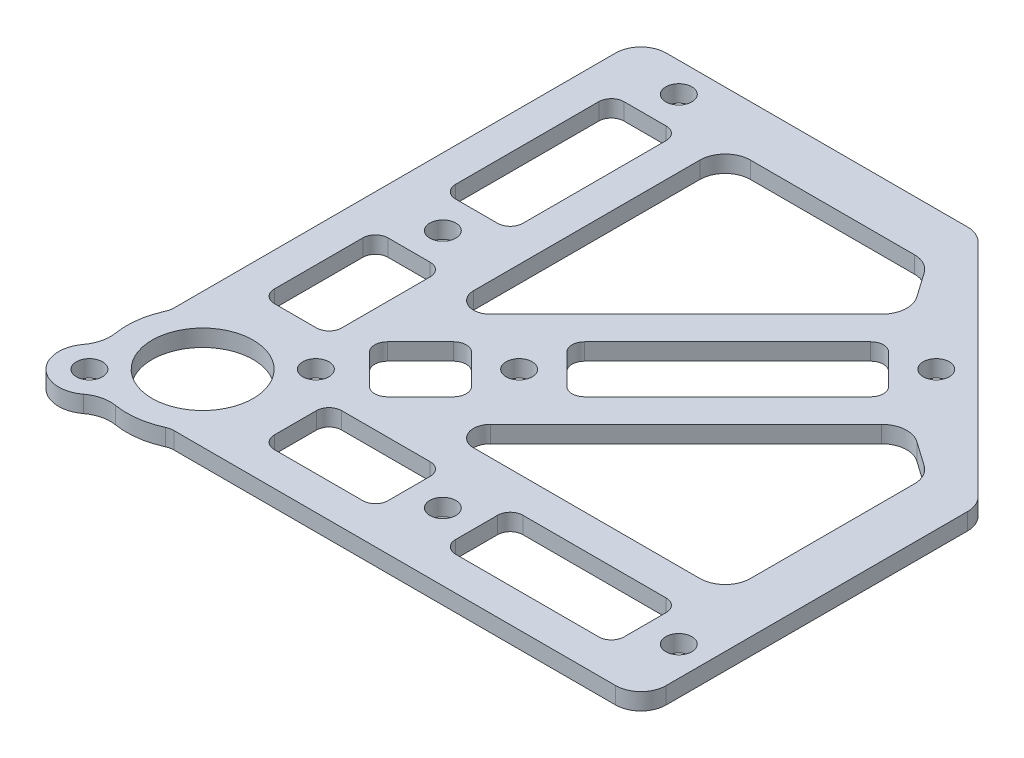
SolidWorks part; units mm, degrees
material "Thornel Mat VMA"
ref_plane "前视基准面" through (0, 0, 0) normal (0, 0, 1) x (1, 0, 0)
ref_plane "上视基准面" through (0, 0, 0) normal (0, 1, 0) x (1, 0, 0)
ref_plane "右视基准面" through (0, 0, 0) normal (1, 0, 0) x (0, 0, -1)
other "Configuration Table"
sketch "草图1" plane through (0, 0, 0) normal (0, 1, 0) x (1, 0, 0)
  line L0 (0, 0) -> (79.3925, 0) construction
  line L1 (0, 0) -> (0, 72.0385) construction
  line L2 (0, 0) -> (60.9542, 60.9542) construction
  line L3 (10.1348, -8) -> (60, -8)
  line L4 (0, 0) -> (-6.7175, 6.7175) construction
  line L5 (60, 32) -> (60, -8)
  line L6 (60, 32) -> (32, 60)
  line L7 (19.3137, 8) -> (54, 8)
  line L8 (54, 8) -> (54, 32)
  line L9 (54, 32) -> (47.7147, 36.401)
  line L10 (47.7147, 36.401) -> (19.3137, 8)
  line L11 (8, 19.3137) -> (8, 54)
  line L12 (32.5, 4) -> (52.5, 4)
  line L13 (32.5, 4) -> (32.5, -4)
  line L14 (32.5, -4) -> (52.5, -4)
  line L15 (52.5, 4) -> (52.5, -4)
  line L16 (11, 4) -> (24.5, 4)
  line L17 (11, 4) -> (11, -4)
  line L18 (11, -4) -> (24.5, -4)
  line L19 (24.5, 4) -> (24.5, -4)
  line L20 (36.401, 47.7147) -> (8, 19.3137)
  line L21 (32, 54) -> (36.401, 47.7147)
  line L22 (8, 54) -> (32, 54)
  line L23 (32, 60) -> (-8, 60)
  line L24 (4, 52.5) -> (-4, 52.5)
  line L25 (-4, 32.5) -> (-4, 52.5)
  line L26 (4, 32.5) -> (4, 52.5)
  line L27 (4, 32.5) -> (-4, 32.5)
  line L28 (4, 24.5) -> (-4, 24.5)
  line L29 (4, 11) -> (4, 24.5)
  line L30 (4, 11) -> (-4, 11)
  line L31 (-4, 11) -> (-4, 24.5)
  line L32 (-8, 10.1348) -> (-8, 60)
  line L33 (18.7764, 24.4332) -> (24.4332, 18.7764)
  line L34 (24.4332, 18.7764) -> (43.5251, 37.8683)
  line L35 (43.5251, 37.8683) -> (37.8683, 43.5251)
  line L36 (37.8683, 43.5251) -> (18.7764, 24.4332)
  line L37 (7.0711, 12.7279) -> (12.7279, 7.0711)
  line L38 (12.7279, 7.0711) -> (18.7764, 13.1195)
  line L39 (18.7764, 13.1195) -> (13.1195, 18.7764)
  line L40 (13.1195, 18.7764) -> (7.0711, 12.7279)
  line L41 (-8, 10.1348) -> (-8, 4.1231)
  line L42 (10.1348, -8) -> (4.1231, -8)
  circle A0 centre (0, 0) radius 6
  circle A1 centre (-6.7175, 6.7175) radius 1.55 construction
  circle A2 centre (6.7175, -6.7175) radius 1.55 construction
  circle A3 centre (56.5, 0) radius 1.55
  circle A4 centre (28.5, 0) radius 1.55
  arc A5 (3.4371, -8.3179) -> (8.3179, -3.4371) centre (6.7175, -6.7175) ccw construction
  circle A6 centre (43.5251, 43.5251) radius 1.55
  circle A7 centre (18.7764, 18.7764) radius 1.55
  circle A8 centre (0, 56.5) radius 1.55
  circle A9 centre (0, 28.5) radius 1.55
  arc A10 (-8.3179, 3.4371) -> (-3.4371, 8.3179) centre (-6.7175, 6.7175) cw construction
  circle A11 centre (0, 0) radius 9
  circle A12 centre (6.7175, 6.7175) radius 1.55
  circle A13 centre (-6.7175, -6.7175) radius 1.55
  circle A14 centre (-6.7175, -6.7175) radius 3.65
  point P41 (46, 46)
  dimension "D1" = 12
  dimension "D5" = 3.1
  dimension "D7" = 3.5
  dimension "D8" = 28
  dimension "D9" = 2.1
  dimension "D10" = 3.5
  dimension "D11" = 35
  dimension "D22" = 18
  dimension "D27" = 11
  dimension "D28" = 14
  dimension "D2" = 45
  dimension "D3" = 8
  dimension "D4" = 9.5
  dimension "D6" = 60
  dimension "D12" = 40
  dimension "D13" = 6
  dimension "D14" = 8
  dimension "D15" = 8
  dimension "D16" = 80
  dimension "D17" = 4
  dimension "D18" = 24
  dimension "D19" = 4
  dimension "D20" = 4
  dimension "D21" = 4
  dimension "D23" = 4
  dimension "D24" = 4
  dimension "D25" = 4
  dimension "D26" = 4
extrude "凸台-拉伸1" add sketch "草图1" along normal blind 2 contours A12 A11 L42 L3 L5 L6 L23 L32 L41 A9 L30 L31 L28 L29 L26 L27 L25 L24 L11 L22 L21 L20 L16 L19 L18 L17 L12 L15 L14 L13 L10 L9 L8 L7 L36 L35 L34 L33 L40 L39 L38 | A14 A11 A12 A0 | A11 A14 A0 A13 | A11 A14 A13
fillet "圆角1" radius 2 4 edges at (8, 1, -19.3137) (19.3137, 1, -8) (4.1231, 1, 8) (-8, 1, -4.1231)
fillet "圆角2" radius 1.5 24 edges at (32.5, 1, 4) (52.5, 1, 4) (52.5, 1, -4) (32.5, 1, -4) (11, 1, 4) (24.5, 1, 4) (24.5, 1, -4) (11, 1, -4) (24.4332, 1, -18.7764) (43.5251, 1, -37.8683) (37.8683, 1, -43.5251) (18.7764, 1, -24.4332) (7.0711, 1, -12.7279) (12.7279, 1, -7.0711) (18.7764, 1, -13.1195) (13.1195, 1, -18.7764) (4, 1, -52.5) (-4, 1, -32.5) (4, 1, -32.5) (-4, 1, -52.5) (4, 1, -11) (4, 1, -24.5) (-4, 1, -11) (-4, 1, -24.5)
fillet "圆角3" radius 3 10 edges at (60, 1, -32) (60, 1, 8) (54, 1, -8) (54, 1, -32) (47.7147, 1, -36.401) (8, 1, -54) (36.401, 1, -47.7147) (32, 1, -54) (32, 1, -60) (-8, 1, -60)
fillet "圆角4" radius 4 2 edges at (-3.4371, 1, 8.3179) (-8.3179, 1, 3.4371)
